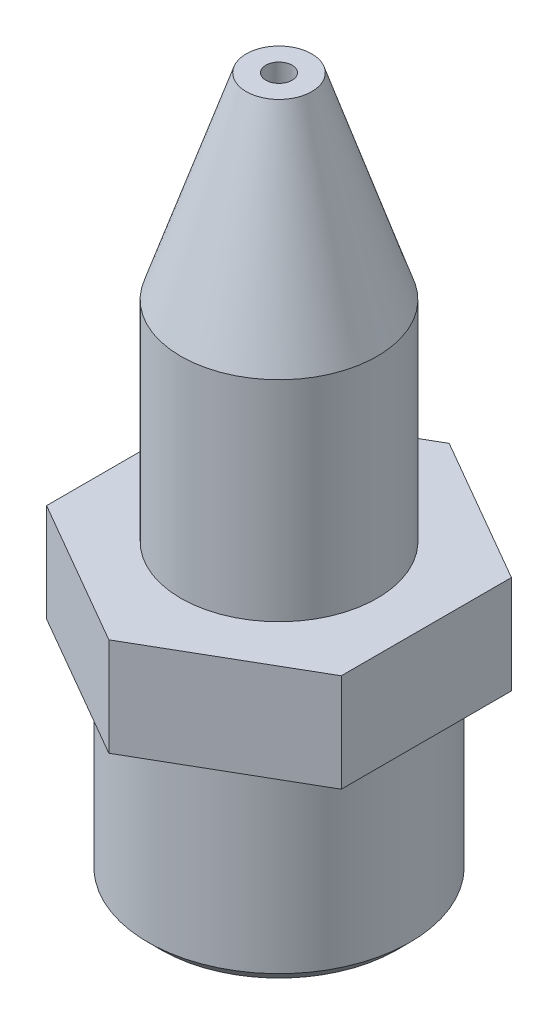
from build123d import *

# Parameters (mm, degrees)
SKETCH1_R           = 1.5
BOSS_EXTRUDE1_DEPTH = 6.2
SKETCH3_R           = 0.2
CUT_EXTRUDE2_DEPTH  = 7.55286197
CHAMFER1_SIZE       = 3
CHAMFER1_SIZE2      = 1
SKETCH5_R           = 0.5
CUT_EXTRUDE3_DEPTH  = 1.5
BOSS_EXTRUDE2_START = 1.5
SKETCH7_R           = 0.5
BOSS_EXTRUDE2_DEPTH = 1.5
BOSS_EXTRUDE3_START = 3
SKETCH8_R           = 2
SKETCH8_R_2         = 0.5
BOSS_EXTRUDE3_DEPTH = 3
CHAMFER4_SIZE       = 0.2


with BuildPart() as part:
    # Sketch1 → Boss-Extrude1 (new body)
    with BuildSketch(Plane(origin=(0, 0, 0), x_dir=(1, 0, 0), z_dir=(0, 1, 0))):
        with Locations(Location((0, 0, 0), (0, 0, 90))):
            Circle(SKETCH1_R)
    extrude(amount=BOSS_EXTRUDE1_DEPTH)

    # Sketch3 → Cut-Extrude2 (cut, through all)
    with BuildSketch(Plane(origin=(0, 6.2, 0), x_dir=(1, 0, 0), z_dir=(0, 1, 0))):
        with Locations(Location((0, 0, 0), (0, 0, 270))):
            Circle(SKETCH3_R)
    extrude(amount=-CUT_EXTRUDE2_DEPTH, mode=Mode.SUBTRACT)

    # Chamfer1
    chamfer1_edges = [part.edges().sort_by_distance(p)[0] for p in [
        (0, 6.2, 1.5),
    ]]
    chamfer1_side = [part.faces().sort_by_distance(p)[0] for p in [
        (0, 3.1, 1.5),
    ]]
    chamfer(chamfer1_edges, length=CHAMFER1_SIZE, length2=CHAMFER1_SIZE2, reference=chamfer1_side[0])

    # Sketch5 → Cut-Extrude3 (cut)
    with BuildSketch(Plane.XZ):
        with Locations(Location((0, 0, 0), (0, 0, 270))):
            Circle(SKETCH5_R)
    extrude(amount=-CUT_EXTRUDE3_DEPTH, mode=Mode.SUBTRACT)

    # Sketch7 → Boss-Extrude2 (add)
    with BuildSketch(Plane.XZ.offset(BOSS_EXTRUDE2_START)):
        Polygon((0, 2.598076211), (-2.25, 1.299038106), (-2.25, -1.299038106), (0, -2.598076211), (2.25, -1.299038106), (2.25, 1.299038106), align=None)
        with Locations(Location((0, 0, 0), (0, 0, 270))):
            Circle(SKETCH7_R, mode=Mode.SUBTRACT)
    extrude(amount=-BOSS_EXTRUDE2_DEPTH)

    # Sketch8 → Boss-Extrude3 (add)
    with BuildSketch(Plane.XZ.offset(1.5).offset(BOSS_EXTRUDE3_START)):
        with Locations(Location((0, 0, 0), (0, 0, 270))):
            Circle(SKETCH8_R)
        with Locations(Location((0, 0, 0), (0, 0, 270))):
            Circle(SKETCH8_R_2, mode=Mode.SUBTRACT)
    extrude(amount=-BOSS_EXTRUDE3_DEPTH)

    # Sketch9 → Cut-Revolve2 (revolve, cut)
    with BuildSketch(Plane.XY, mode=Mode.PRIVATE) as cut_revolve2_sk:
        Polygon((0.2, 6.2), (1.1, -4.5), (0, -4.5), (0, 6.2), align=None)
    revolve(cut_revolve2_sk.sketch.rotate(Axis((0, -1009.643261514, 0), (0, 1, 0)), 90), axis=Axis((0, -1009.643261514, 0), (0, 1, 0)), mode=Mode.SUBTRACT)

    # Chamfer4
    chamfer4_edges = [part.edges().sort_by_distance(p)[0] for p in [
        (0, -4.5, 2),
    ]]
    chamfer(chamfer4_edges, length=CHAMFER4_SIZE)


solid = part.part
